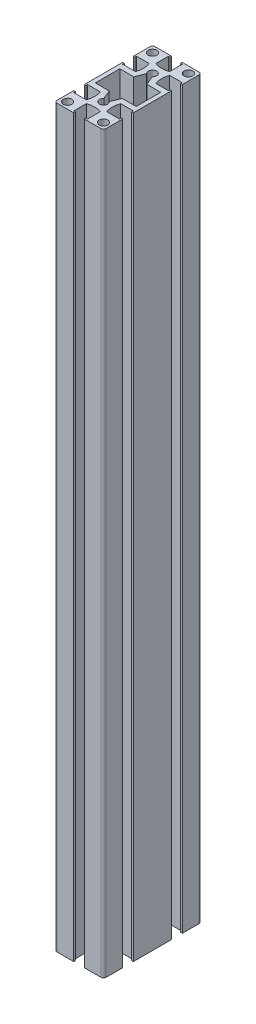
SolidWorks part; units mm, degrees
ref_plane "前视基准面" through (0, 0, 0) normal (0, 0, 1) x (1, 0, 0)
ref_plane "上视基准面" through (0, 0, 0) normal (0, 1, 0) x (1, 0, 0)
ref_plane "右视基准面" through (0, 0, 0) normal (1, 0, 0) x (0, 0, -1)
sketch "草图1" plane through (0, 0, 0) normal (0, 0, 1) x (1, 0, 0)
  line L9 (0, 0) -> (0, 450)
  dimension "D1" = 450
other "工业铝型材 30 X 60G X R1.5(1)"
ref_plane "基准面1" through (0, 0, 0) normal (0, 1, 0) x (-1, 0, 0)
sketch "Sketch1" plane through (0, 0, 0) normal (0, 1, 0) x (-1, 0, 0)
  line L0 (-3.25, 30) -> (-3.25, 29)
  line L1 (-13.5, 30) -> (-3.25, 30)
  line L2 (-15, 28.5) -> (-15, 18.25)
  line L3 (-13.5, -30) -> (-3.25, -30)
  line L4 (15, 28.5) -> (15, 18.25)
  line L5 (-12.5, 7.5) -> (-4, 7.5)
  line L6 (-12.5, 7.5) -> (-12.5, -7.5)
  line L7 (-12.5, -7.5) -> (-4, -7.5)
  line L8 (0, 30) -> (0, 0) construction
  line L9 (0, 0) -> (15, 0) construction
  line L10 (12.5, 7.5) -> (12.5, -7.5)
  line L11 (-3.25, 29) -> (-4.25, 29)
  line L12 (-4.25, 29) -> (-4.25, 21.2778)
  line L13 (-11, 26) -> (-15, 30) construction
  line L14 (4.25, 29) -> (4.25, 21.2778)
  line L15 (3.25, 29) -> (4.25, 29)
  line L16 (3.25, 30) -> (3.25, 29)
  line L17 (3.25, 30) -> (13.5, 30)
  line L18 (-1.6656, 13.1357) -> (-4, 7.5)
  line L19 (1.6656, 13.1357) -> (4, 7.5)
  line L20 (4, 7.5) -> (12.5, 7.5)
  line L21 (1.6656, -13.1357) -> (4, -7.5)
  line L22 (-1.6656, -13.1357) -> (-4, -7.5)
  line L23 (4, -7.5) -> (12.5, -7.5)
  line L24 (15, 18.25) -> (14, 18.25)
  line L25 (14, 18.25) -> (14, 19.25)
  line L26 (14, 19.25) -> (6.2778, 19.25)
  line L27 (14, 10.75) -> (6.2778, 10.75)
  line L28 (14, 11.75) -> (14, 10.75)
  line L29 (15, 11.75) -> (14, 11.75)
  line L30 (3.25, 0) -> (3.25, 1) [skipped]
  line L31 (3.25, 1) -> (4.25, 1) [skipped]
  line L32 (4.25, 1) -> (4.25, 8.7222) [skipped]
  line L33 (-4.25, 1) -> (-4.25, 8.7222) [skipped]
  line L34 (-3.25, 1) -> (-4.25, 1) [skipped]
  line L35 (-3.25, 0) -> (-3.25, 1) [skipped]
  line L36 (-15, 11.75) -> (-14, 11.75)
  line L37 (-14, 11.75) -> (-14, 10.75)
  line L38 (-14, 10.75) -> (-6.2778, 10.75)
  line L39 (-14, 19.25) -> (-6.2778, 19.25)
  line L40 (-14, 18.25) -> (-14, 19.25)
  line L41 (-15, 18.25) -> (-14, 18.25)
  line L42 (-15, 11.75) -> (-15, -11.75)
  line L43 (15, 11.75) -> (15, -11.75)
  line L44 (-15, -18.25) -> (-14, -18.25)
  line L45 (-14, -18.25) -> (-14, -19.25)
  line L46 (-14, -19.25) -> (-6.2778, -19.25)
  line L47 (-14, -10.75) -> (-6.2778, -10.75)
  line L48 (-14, -11.75) -> (-14, -10.75)
  line L49 (-15, -11.75) -> (-14, -11.75)
  line L50 (15, -11.75) -> (14, -11.75)
  line L51 (14, -11.75) -> (14, -10.75)
  line L52 (14, -10.75) -> (6.2778, -10.75)
  line L53 (14, -19.25) -> (6.2778, -19.25)
  line L54 (14, -18.25) -> (14, -19.25)
  line L55 (15, -18.25) -> (14, -18.25)
  line L56 (3.25, -30) -> (3.25, -29)
  line L57 (3.25, -29) -> (4.25, -29)
  line L58 (4.25, -29) -> (4.25, -21.2778)
  line L59 (-4.25, -29) -> (-4.25, -21.2778)
  line L60 (-3.25, -29) -> (-4.25, -29)
  line L61 (-3.25, -30) -> (-3.25, -29)
  line L62 (3.25, -30) -> (13.5, -30)
  line L63 (-15, -18.25) -> (-15, -28.5)
  line L64 (15, -18.25) -> (15, -28.5)
  arc A0 (-4.25, 21.2778) -> (4.25, 21.2778) centre (0, 32.5) ccw
  circle A1 centre (-11, 26) radius 2.65
  circle A2 centre (11, 26) radius 2.65
  arc A3 (-15, 28.5) -> (-13.5, 30) centre (-13.5, 28.5) cw
  arc A4 (15, 28.5) -> (13.5, 30) centre (13.5, 28.5) ccw
  arc A5 (15, -28.5) -> (13.5, -30) centre (13.5, -28.5) cw
  arc A6 (-13.5, -30) -> (-15, -28.5) centre (-13.5, -28.5) cw
  arc A7 (1.6656, 13.1357) -> (-1.6656, 13.1357) centre (0, 15) ccw
  arc A8 (-1.6656, -13.1357) -> (1.6656, -13.1357) centre (0, -15) ccw
  arc A9 (6.2778, 19.25) -> (6.2778, 10.75) centre (17.5, 15) ccw
  arc A10 (4.25, 8.7222) -> (-4.25, 8.7222) centre (0, -2.5) ccw [skipped]
  arc A11 (-6.2778, 10.75) -> (-6.2778, 19.25) centre (-17.5, 15) ccw
  arc A12 (-6.2778, -10.75) -> (-6.2778, -19.25) centre (-17.5, -15) cw
  arc A13 (6.2778, -19.25) -> (6.2778, -10.75) centre (17.5, -15) cw
  circle A14 centre (11, -26) radius 2.65
  arc A15 (-4.25, -21.2778) -> (4.25, -21.2778) centre (0, -32.5) cw
  circle A16 centre (-11, -26) radius 2.65
  point P102 (15, -30)
  point P103 (-15, -30)
  point P104 (0, 0)
  dimension "D1" = 60
  dimension "D2" = 30
  dimension "D3" = 15
  dimension "D4" = 2.5
  dimension "D5" = 6.5
  dimension "D6" = 8.5
  dimension "D7" = 12
  dimension "D8" = 1
  dimension "D10" = 5.3
  dimension "D11" = 4
  dimension "D12" = 1.5
  dimension "D13" = 5
  dimension "D14" = 30
  dimension "D9" = 9.5
  dimension "D15" = 45
  dimension "D16" = 8
